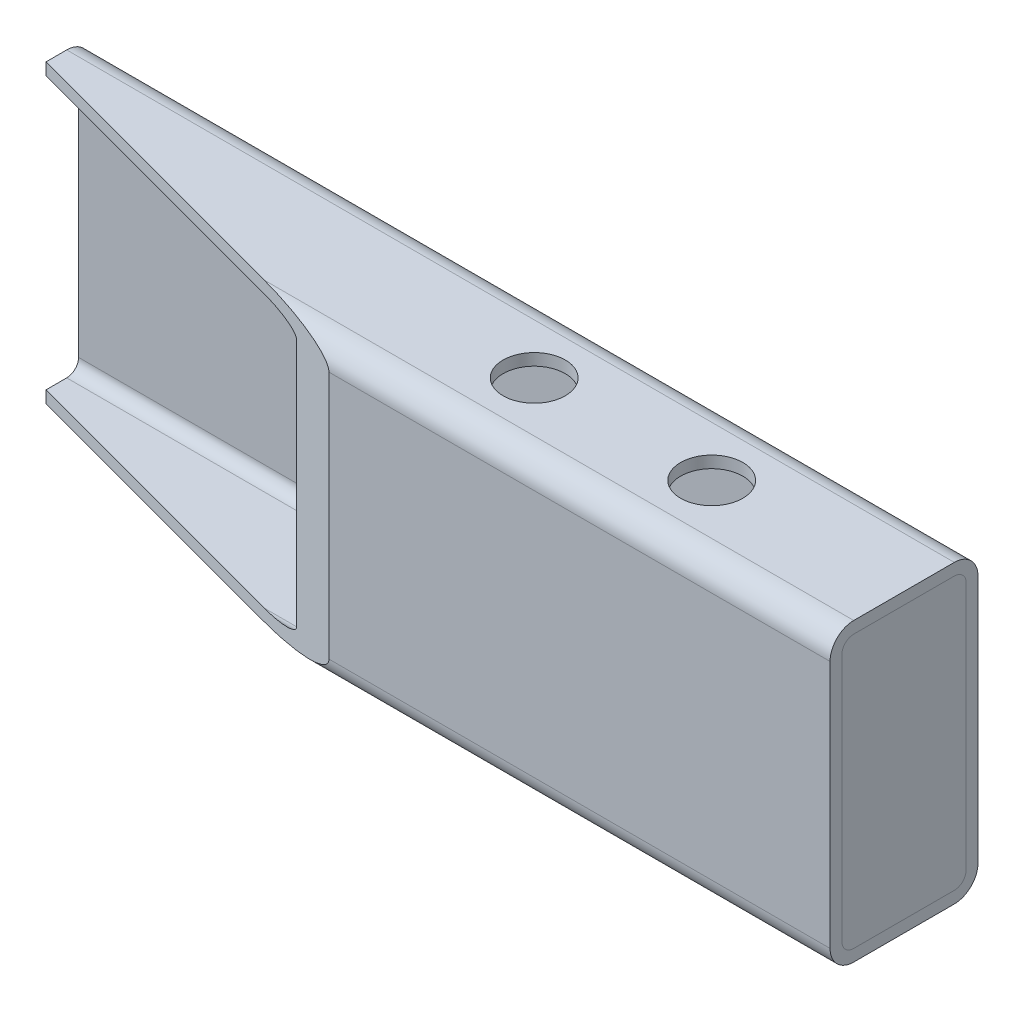
from build123d import *

# Parameters (mm, degrees)
RECTANGULAR_TUBE_100_X_50_X_4_1_DEPTH = 300
CUT_EXTRUDE1_REACH                    = 319.214
SKETCH2_R                             = 10.5
BOSS_EXTRUDE1_DEPTH                   = 25


with BuildPart() as part:
    # Sketch1 → Rectangular tube 100 X 50 X 4 (1) (new body)
    with BuildSketch(Plane(origin=(0, 0, 0), x_dir=(0, 0, -1), z_dir=(1, 0, 0))):
        with BuildLine():
            Line((-17, -50), (17, -50))
            ThreePointArc((17, -50), (22.656854249, -47.656854249), (25, -42))
            Line((25, -42), (25, 42))
            ThreePointArc((25, 42), (22.656854249, 47.656854249), (17, 50))
            Line((17, 50), (-17, 50))
            ThreePointArc((-17, 50), (-22.656854249, 47.656854249), (-25, 42))
            Line((-25, 42), (-25, -42))
            ThreePointArc((-25, -42), (-22.656854249, -47.656854249), (-17, -50))
        make_face()
        with BuildLine():
            Line((-17, -46), (17, -46))
            ThreePointArc((17, -46), (19.828427125, -44.828427125), (21, -42))
            Line((21, -42), (21, 42))
            ThreePointArc((21, 42), (19.828427125, 44.828427125), (17, 46))
            Line((17, 46), (-17, 46))
            ThreePointArc((-17, 46), (-19.828427125, 44.828427125), (-21, 42))
            Line((-21, 42), (-21, -42))
            ThreePointArc((-21, -42), (-19.828427125, -44.828427125), (-17, -46))
        make_face(mode=Mode.SUBTRACT)
    extrude(amount=RECTANGULAR_TUBE_100_X_50_X_4_1_DEPTH)

    # Cut-Extrude1: up to this face of the body (flat: up to its plane)
    cut_extrude1_end = Plane(part.part.faces().sort_by_distance((150, 50, 0))[0])
    # Sketch2 → Cut-Extrude1 (cut, up to the picked face)
    with BuildSketch(Plane.XZ.offset(50), mode=Mode.PRIVATE) as cut_extrude1_sk1:
        with Locations(Location((235, 0, 0), (0, 0, 270))):
            Circle(SKETCH2_R)
    cut_extrude1_tool1 = split(extrude(cut_extrude1_sk1.sketch, amount=-CUT_EXTRUDE1_REACH, mode=Mode.PRIVATE), bisect_by=cut_extrude1_end, keep=Keep.BOTH, mode=Mode.PRIVATE)
    # Sketch2 → Cut-Extrude1 (cut, up to the picked face)
    with BuildSketch(Plane.XZ.offset(50), mode=Mode.PRIVATE) as cut_extrude1_sk2:
        with Locations(Location((175, 0, 0), (0, 0, 270))):
            Circle(SKETCH2_R)
    cut_extrude1_tool2 = split(extrude(cut_extrude1_sk2.sketch, amount=-CUT_EXTRUDE1_REACH, mode=Mode.PRIVATE), bisect_by=cut_extrude1_end, keep=Keep.BOTH, mode=Mode.PRIVATE)
    # Sketch2 → Cut-Extrude1 (cut, up to the picked face)
    with BuildSketch(Plane.XZ.offset(50), mode=Mode.PRIVATE) as cut_extrude1_sk3:
        Polygon((0, -10), (130.621778265, 25), (0, 25), align=None)
    cut_extrude1_tool3 = split(extrude(cut_extrude1_sk3.sketch, amount=-CUT_EXTRUDE1_REACH, mode=Mode.PRIVATE), bisect_by=cut_extrude1_end, keep=Keep.BOTH, mode=Mode.PRIVATE)
    add(cut_extrude1_tool1.solids().sort_by(Axis((235, -50, 0), (0, 1, 0)))[0], mode=Mode.SUBTRACT)
    add(cut_extrude1_tool2.solids().sort_by(Axis((175, -50, 0), (0, 1, 0)))[0], mode=Mode.SUBTRACT)
    add(cut_extrude1_tool3.solids().sort_by(Axis((43.540593, -50, 13.333333), (0, 1, 0)))[0], mode=Mode.SUBTRACT)


with BuildPart() as body_2:
    # Sketch3 → Boss-Extrude1 (new body)
    with BuildSketch(Plane(origin=(300, 0, 0), x_dir=(0, 0, -1), z_dir=(1, 0, 0))):
        with BuildLine():
            Line((-17, 46), (17, 46))
            ThreePointArc((17, 46), (19.828427125, 44.828427125), (21, 42))
            Line((21, 42), (21, -42))
            ThreePointArc((21, -42), (19.828427125, -44.828427125), (17, -46))
            Line((17, -46), (-17, -46))
            ThreePointArc((-17, -46), (-19.828427125, -44.828427125), (-21, -42))
            Line((-21, -42), (-21, 42))
            ThreePointArc((-21, 42), (-19.828427125, 44.828427125), (-17, 46))
        make_face()
    extrude(amount=-BOSS_EXTRUDE1_DEPTH)


solid = Compound([part.part, body_2.part])
